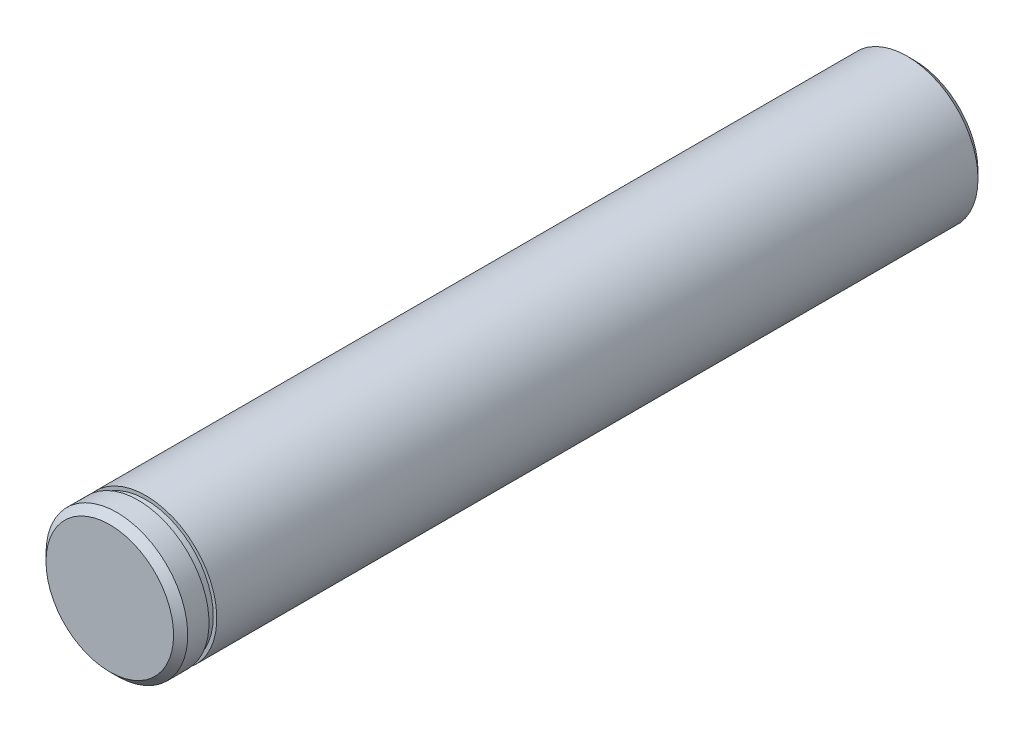
from build123d import *

# Parameters (mm, degrees)
SKETCH_1_R             = 10
EXTRUDE_1_DEPTH        = 113.5
SKETCH_2_W             = 0.5
SKETCH_2_H             = 1.1
CHAMFER_1_SIZE         = 1
HOLE_WIZARD_M6_1_D     = 5
HOLE_WIZARD_M6_1_DEPTH = 21


with BuildPart() as part:
    # 草图1 → 凸台-拉伸1 (new body)
    with BuildSketch(Plane.XY):
        with Locations(Location((0, 0, 0), (0, 0, 180))):
            Circle(SKETCH_1_R)
    extrude(amount=EXTRUDE_1_DEPTH)

    # 草图2 → 切除-旋转1 (revolve, cut)
    with BuildSketch(Plane(origin=(0, 0, 0), x_dir=(1, 0, 0), z_dir=(0, 1, 0)), mode=Mode.PRIVATE) as cut_revolve_1_sk:
        with Locations((9.75, -108.95)):
            Rectangle(SKETCH_2_W, SKETCH_2_H)
    revolve(cut_revolve_1_sk.sketch.rotate(Axis((0, 0, 113.5), (0, 0, -1)), 180), axis=Axis((0, 0, 113.5), (0, 0, -1)), mode=Mode.SUBTRACT)

    # 倒角1
    chamfer_1_edges = [part.edges().sort_by_distance(p)[0] for p in [
        (10, 0, 0),
        (10, 0, 113.5),
    ]]
    chamfer(chamfer_1_edges, length=CHAMFER_1_SIZE)

    # M6 螺纹孔1
    with Locations(Plane(origin=(0, 0, 0), x_dir=(-1, 0, 0), z_dir=(0, 0, -1))):
        with Locations((0, 0)):
            Hole(HOLE_WIZARD_M6_1_D / 2, depth=HOLE_WIZARD_M6_1_DEPTH)


solid = part.part
